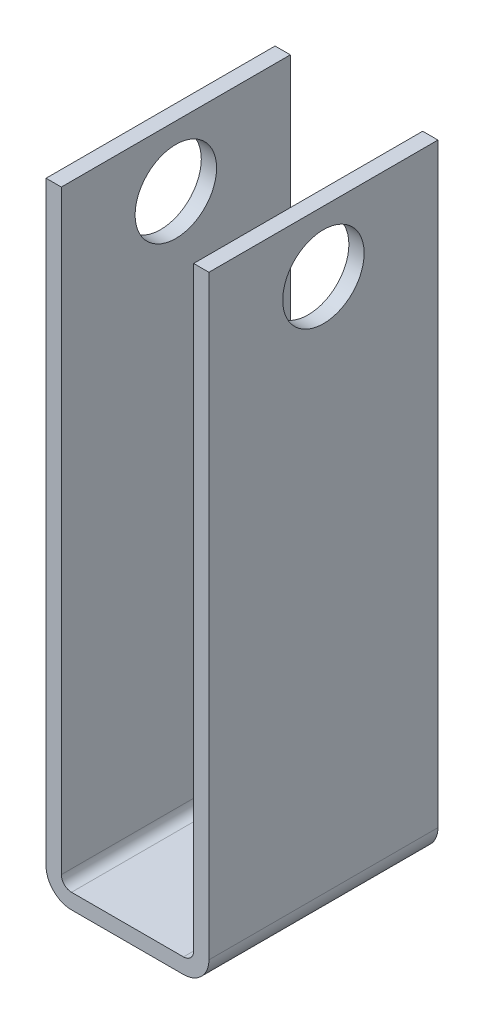
SolidWorks part; units mm, degrees
ref_plane "Front Plane" through (0, 0, 0) normal (0, 0, 1) x (1, 0, 0)
ref_plane "Top Plane" through (0, 0, 0) normal (0, 1, 0) x (1, 0, 0)
ref_plane "Right Plane" through (0, 0, 0) normal (1, 0, 0) x (0, 0, -1)
sketch "Sketch1" plane through (0, 0, 0) normal (0, 0, 1) x (1, 0, 0)
  line L0 (0, 0) -> (0, -117)
  line L1 (5, -122) -> (27, -122)
  line L2 (32, -117) -> (32, 0)
  line L3 (3, 0) -> (3, -117)
  line L4 (5, -119) -> (27, -119)
  line L5 (29, -117) -> (29, 0)
  line L6 (3, 0) -> (0, 0)
  line L7 (29, 0) -> (32, 0)
  arc A0 (27, -122) -> (32, -117) centre (27, -117) ccw
  arc A1 (0, -117) -> (5, -122) centre (5, -117) ccw
  arc A2 (3, -117) -> (5, -119) centre (5, -117) ccw
  arc A3 (27, -119) -> (29, -117) centre (27, -117) ccw
  point P8 (32, -122)
  point P11 (0, -122)
  dimension "D3" = 5
  dimension "D1" = 32
  dimension "D2" = 122
  dimension "D4" = 3
extrude "Boss-Extrude1" add sketch "Sketch1" along normal blind 45
sketch "Sketch2" plane through (32, 0, 0) normal (1, 0, 0) x (0, 0, -1)
  line L0 (0, -117) -> (0, 0) construction
  line L1 (-45, 0) -> (0, 0) construction
  circle A0 centre (-22.5, -12) radius 8
  dimension "D1" = 16
  dimension "D2" = 22.5
  dimension "D3" = 12
extrude "Cut-Extrude1" cut sketch "Sketch2" against normal through all
